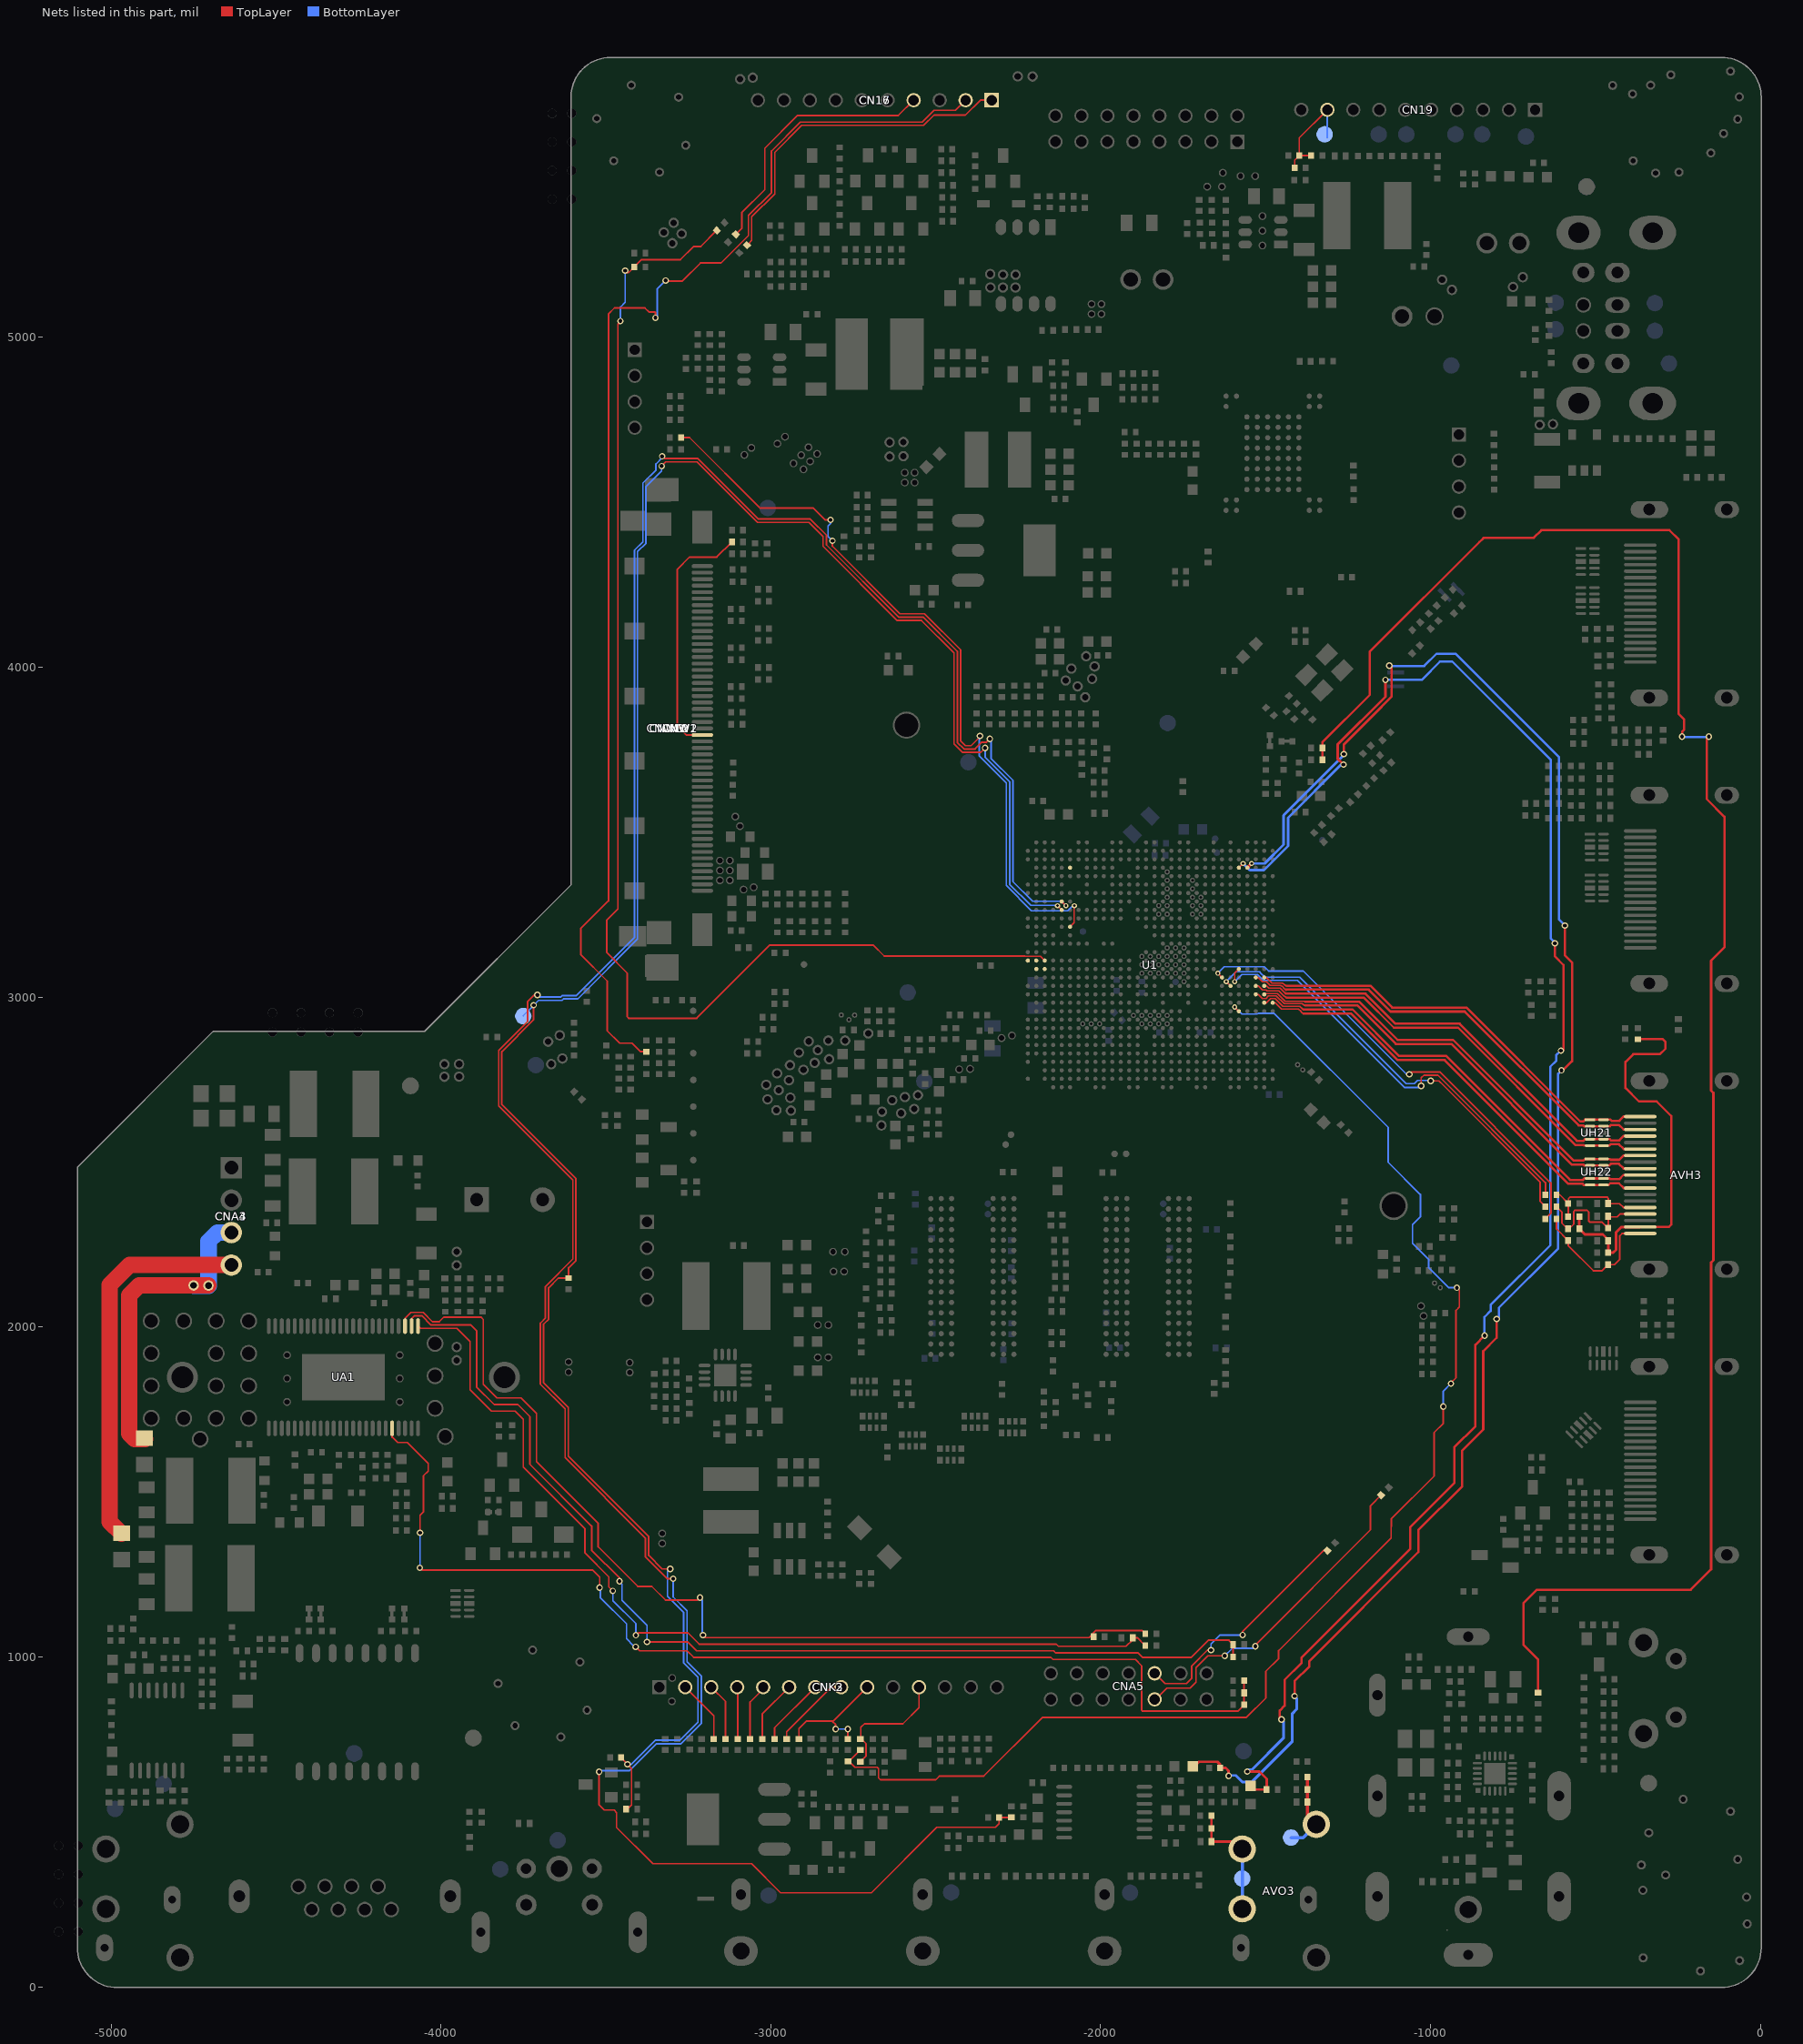
[diagram p0: the nets of this part, all layers, seen from the top]
# Altium PCB MISC86290.PcbDoc (part 23 of 31)
Units mil, origin at the board's own origin, x right, y up, seen from the top; angles counter-clockwise.
Board outline 5104.71 x 5851.49 mil, 2 copper layers (TopLayer, BottomLayer), stack 61.855 mil thick; 1026 components, 667 nets, 4280 pads, 2294 vias.

## Via types
v1: diameter 19.68, hole 11.81, TopLayer to BottomLayer, tented both sides, 1189 vias
v2: diameter 19.68/19.68 (per signal layer), hole 11.81, TopLayer to BottomLayer, tented both sides, 366 vias
v3: diameter 15.75, hole 7.87, TopLayer to BottomLayer, tented both sides, 348 vias
v4: diameter 23.62, hole 15.75, TopLayer to BottomLayer, tented both sides, 309 vias
v5: diameter 15.75/15.75 (per signal layer), hole 7.87, TopLayer to BottomLayer, tented both sides, 59 vias
v6: diameter 24/24 (per signal layer), hole 16, TopLayer to BottomLayer, tented both sides, 23 vias

## Nets (pads, with @x,y where several pads share a name; then routed paths per layer and width w, separated by ;. In a path a pad name is that pad's centre, name@x,y a point inside that pad or via, vN(x,y) a via of type N, cw(c..) or ccw(c..) an arc to the next point about the centre after c; other vN are vias at no path point) (continued)
HDMID-HOTPLUG: RH21.1 U1.P7 | length 1429.1
  TopLayer w3.94: v3(-1645,3072.44) U1.P7@-1632.2,3059.65
  TopLayer w5: v1(-1064.29,2766) -1056.94,2773.35 -972.21,2773.35 -635,2436.15 -635,2344.73 RH21.1@-651.73,2328
  BottomLayer w3.94: v3(-1645,3072.44) -1625.32,3092.13 -1503.82,3092.13 -1501.52,3089.83
  BottomLayer w5: -1501.52,3089.83 -1490.8,3079.11 -1385.61,3079.11 -1072.49,2766 v1(-1064.29,2766)
HDMID-RX0N: AVH3.9 U1.M3 UH22.2 UH22.7 | length 1414.2
  TopLayer w3.94: U1.M3@-1529.84,3008.46 -1522.51,3008.46 -1509.72,2995.67 -1499.19,2995.67 -1491.32,3003.54 -1467.83,3003.54 -1444.21,2979.92 -1391.46,2979.92 cw(c-1391.46,2970.05) -1386.96,2978.84 ; -1384.48,2977.03 ccw(c-1391.46,2970.05) -1385.46,2977.89 ; -1378.29,2975.88 cw(c-1378.29,2989.68) -1385.46,2977.89 ; -1373,2974.58 -1382.71,2974.58 -1386.96,2978.84 ; -1386.96,2978.84 cw(c-1391.46,2970.05) -1386.48,2978.57 ; -1386.48,2978.57 cw(c-1391.46,2970.05) -1385.46,2977.89 ; -1386.48,2978.57 ccw(c-1378.29,2989.68) -1385.46,2977.89
  TopLayer w7: -1380.76,2974.58 -1373,2974.58 -1221.44,2974.58 -1105.21,2858.35 -937,2858.35 -570.89,2492.25 -537,2492.25 -534.44,2489.69 UH22.2@-516.47,2489.69 UH22.7@-475.53,2489.68 -458.13,2489.68 -453,2494.81 -428.92,2494.81 -414.43,2480.32 AVH3.9@-364.47,2480.32
HDMID-RX0P: AVH3.7 U1.M2 UH22.1 UH22.8 | length 1366.6
  TopLayer w3.94: U1.M2@-1504.25,3008.46 -1503.19,3007.4 -1499.17,3011.42 -1463.9,3011.42 -1440.39,2987.91 -1386.58,2987.91 ; -1381.07,2985.63 ccw(c-1386.58,2980.12) -1386.58,2987.91 ; -1379.37,2987.91 -1386.58,2987.91
  TopLayer w7: -1379.9,2986.58 -1216.47,2986.58 -1100.24,2870.35 -932.03,2870.35 -565.92,2504.25 -537,2504.25 -531.87,2509.37 UH22.1@-516.47,2509.37 UH22.8@-475.53,2509.37 -456.56,2509.37 -454,2506.81 -428.08,2506.81 -415.2,2519.69 AVH3.7@-364.47,2519.69
HDMID-RX1N: AVH3.6 U1.N3 UH21.4 UH21.5 | length 1388.1
  TopLayer w3.94: U1.N3@-1529.84,3034.06 -1522.05,3034.06 -1509.64,3021.65 -1498.15,3021.65 -1495.79,3019.29 -1459.96,3019.29 -1443.48,3002.81 ; -1436.82,3000.05 cw(c-1436.82,3009.47) -1443.48,3002.81 ; -1436.25,2999.03 -1439.7,2999.03 ; -1435.7,2997.12 cw(c-1435.7,3002.16) -1439.27,2998.6 -1439.7,2999.03 ; -1443.48,3002.81 -1441.48,3000.81 ; -1441.48,3000.81 -1439.7,2999.03 ; -1441.48,3000.81 -1439.7,2999.03
  TopLayer w7: -1436.25,2998.58 -1202.44,2998.58 -1111.21,2907.35 -916.7,2907.35 -561.54,2552.19 -537,2552.19 -534.44,2549.63 UH21.4@-516.47,2549.63 UH21.5@-475.53,2549.63 -458.24,2549.63 -454,2553.87 -428.92,2553.87 -414.43,2539.37 AVH3.6@-364.47,2539.37
HDMID-RX1P: AVH3.4 U1.N2 UH21.3 UH21.6 | length 1352.1
  TopLayer w3.94: U1.N2@-1504.25,3034.06 -1497.85,3034.06 -1490.96,3027.17 -1456.02,3027.17 -1444.03,3015.17 ; -1436.96,3009.16 cw(c-1436.96,3011.72) -1438.76,3009.9 -1444.02,3015.16 ccw(c-1436.54,3022.66) -1436.54,3012.07
  TopLayer w7: -1437,3010.58 -1197.47,3010.58 -1106.24,2919.35 -911.73,2919.35 -556.57,2564.19 -537,2564.19 -531.87,2569.32 UH21.3@-516.47,2569.32 UH21.6@-475.53,2569.32 -456.45,2569.32 -453,2565.87 -428.08,2565.87 -415.2,2578.74 AVH3.4@-364.47,2578.74
HDMID-RX2N: AVH3.3 U1.P3 UH21.2 UH21.7 | length 1380.6
  TopLayer w3.94: U1.P3@-1529.84,3059.65 -1522.81,3059.65 -1510.01,3046.85 -1497.85,3046.85 -1486.04,3035.04 -1455.54,3035.04 cw(c-1455.54,3026.7) -1449.64,3032.6 -1444.88,3027.84 ; -1436.53,3021.03 -1438.08,3021.03 -1444.88,3027.84 ; -1444.88,3027.84 ccw(c-1435.69,3037.03) -1435.69,3024.03 cw(c-1435.69,3037.03) -1444.88,3027.84
  TopLayer w7: -1436.53,3022.58 -1187.44,3022.58 -1121.21,2956.35 -896.41,2956.35 -551.3,2611.24 -537,2611.24 -534.44,2608.68 UH21.2@-516.47,2608.68 UH21.7@-475.53,2608.68 -456.93,2608.68 -452.69,2612.92 -428.92,2612.92 -414.43,2598.43 AVH3.3@-364.47,2598.43
HDMID-RX2P: AVH3.1 U1.P2 UH21.1 UH21.8 | length 1355.8
  TopLayer w3.94: U1.P2@-1504.25,3059.65 -1497.85,3059.65 -1481.12,3042.91 -1454.24,3042.91 cw(c-1454.24,3028.21) -1443.85,3038.61 ; -1439.98,3034.74 -1443.83,3038.6 ; -1437.69,3036.06 cw(c-1437.69,3044.76) -1443.83,3038.6 ; -1435,3034.58 -1439.81,3034.58 ; -1432.87,3036.02 -1437.6,3036.02 cw(c-1437.6,3044.85) -1443.83,3038.6 ; -1432.11,3033.89 cw(c-1433.73,3035.51) -1433.73,3033.22 -1436.3,3033.22 cw(c-1436.3,3038.43) -1439.81,3034.58 ; -1439.81,3034.58 cw(c-1436.3,3038.43) -1439.97,3034.74 -1439.82,3034.58
  TopLayer w7: -1435,3034.58 -1182.47,3034.58 -1116.24,2968.35 -891.44,2968.35 -546.33,2623.24 -537,2623.24 -531.87,2628.37 UH21.1@-516.47,2628.37 UH21.8@-475.53,2628.37 -454.45,2628.37 -451,2624.92 -428.08,2624.92 -415.2,2637.8 AVH3.1@-364.47,2637.8
HDMID-RXCKN: AVH3.12 U1.L1 UH22.4 UH22.5 | length 1358.7
  TopLayer w3.94: U1.L1@-1478.66,2982.87 -1470.79,2982.87 -1452.09,2964.17 -1400.91,2964.17 -1394.59,2957.86 -1391.54,2954.81 ; -1386.18,2949.44 -1391.53,2954.8 ; -1386.17,2949.44 ccw(c-1385.37,2950.25) -1385.37,2949.11 ; -1384.88,2952.05 cw(c-1384.88,2961.47) -1391.53,2954.8
  TopLayer w7: -1385,2950.58 -1241.11,2950.58 -1099.88,2809.35 -957.29,2809.35 -581.94,2434 -539,2434 -535.63,2430.63 UH22.4@-516.47,2430.63 UH22.5@-475.53,2430.63 -460.13,2430.63 -455,2435.76 -428.92,2435.76 -414.43,2421.26 AVH3.12@-364.47,2421.26
HDMID-RXCKP: AVH3.10 U1.L2 UH22.3 UH22.6 | length 1391.5
  TopLayer w3.94: U1.L2@-1504.25,2982.87 -1503.66,2982.28 -1498.15,2982.28 -1484.76,2995.67 -1471.77,2995.67 -1448.15,2972.05 -1396.55,2972.05 -1391.62,2967.12 ; -1387.08,2962.58 -1387.66,2963.16 ; -1384.18,2964.04 cw(c-1384.18,2974.56) -1391.62,2967.12 ; -1382.47,2961.01 cw(c-1382.47,2968.35) -1387.66,2963.16 ; -1391.62,2967.12 -1387.66,2963.16
  TopLayer w7: -1383.12,2962.58 -1236.14,2962.58 -1094.91,2821.35 -952.32,2821.35 -576.97,2446 -538,2446 -533.69,2450.32 UH22.3@-516.47,2450.32 UH22.6@-475.53,2450.32 -457.56,2450.32 -455,2447.76 -428.08,2447.76 -415.2,2460.63 AVH3.10@-364.47,2460.63
HDMID-SCL_IC: RH25.2 U1.R5 | length 1337.6
  TopLayer w3.94: v3(-1593.82,3046.85) -1593.82,3072.44 U1.R5@-1581.02,3085.24
  TopLayer w5: v1(-1028.5,2731) -1028.5,2755.35 -1020.5,2763.35 -977.38,2763.35 -651.73,2437.7 RH25.2@-651.73,2401
  BottomLayer w3.94: v3(-1593.82,3046.85) -1572.05,3068.61 -1525.31,3068.61 ; -1525.2,3068.5 -1522.25,3065.55
  BottomLayer w5: -1522.25,3065.55 -1507.42,3050.73 -1403.73,3050.73 -1079.3,2726.3 -1033.2,2726.3 v1(-1028.5,2731)
HDMID-SDA_IC: RH26.2 U1.N6 | length 1335
  TopLayer w3.94: v3(-1619.41,3046.85) U1.N6@-1606.61,3034.06
  TopLayer w5: v1(-999.5,2746) -974.17,2746 -961.17,2733 -668.09,2439.92 -668.09,2380.75 ; -667.73,2381 RH26.2@-651.73,2365
  BottomLayer w3.94: v3(-1619.41,3046.85) -1589.81,3076.45 -1518.14,3076.45 -1514.72,3073.03
  BottomLayer w5: -1514.72,3073.03 -1501.88,3060.19 -1396.19,3060.19 -1073.7,2737.7 -1049.07,2737.7 -1039.53,2747.24 -1000.74,2747.24 v1(-999.5,2746)
HDMID_5V: AVH3.18 CH22.1 DH22.K RH22.2 RH23.2 RH24.2 | length 1259.9
  TopLayer w7: RH22.2@-372,2872.27 -296.27,2872.27 -288,2864 -288,2844 -305,2827 -385.44,2827 -409,2803.44 -409,2724.56 -368.44,2684 -314.79,2684 -270.66,2639.86 -270.66,2310.34 -277.85,2303.15 AVH3.18@-364.47,2303.15
  TopLayer w8: RH24.2@-549.27,2334 RH23.2@-549.27,2298 -532.27,2281 -478,2281 -461.27,2264.27 DH22.K@-461.27,2261 CH22.1@-461.27,2226 -446,2226 -438,2234 -438,2287 -421.85,2303.15 AVH3.18@-364.47,2303.15
HDMID_HPD: AVH3.19 CH21.1 DH21.K RH21.2 | length 434.3
  TopLayer w5: RH21.2@-618.27,2328 -618.27,2297.54 CH21.1@-582.73,2262 -582.73,2246.71 -506.7,2170.67 -479.59,2170.67 DH21.K@-461.27,2189 -442.57,2189 -426.5,2205.07 -426.5,2276.5 -419.53,2283.47 AVH3.19@-364.47,2283.47
HDMID_SCL: AVH3.15 CH24.1 DH24.K RH24.1 RH25.1 | length 343.5
  TopLayer w5: RH25.1@-618.27,2401 -608.63,2401 -582.73,2375.1 CH24.1@-582.73,2374 ; RH24.1@-582.73,2334 CH24.1@-582.73,2373 ; CH24.1@-581.73,2374 -581.73,2389.27 -577,2394 -465,2394 -461.27,2390.27 DH24.K@-461.27,2374 -427,2374 -415.21,2362.21 AVH3.15@-364.47,2362.21
HDMID_SDA: AVH3.16 CH23.1 DH23.K RH23.1 RH26.1 | length 426.3
  TopLayer w5: RH26.1@-618.27,2365 -601.91,2348.64 -601.91,2315.18 -583.73,2297 RH23.1@-582.73,2296 ; RH23.1@-579,2296 -579,2298 -579,2299 -566,2312 -566,2350 -562,2354 -526,2354 -520,2348 -520,2321 -516.67,2317.67 -479.67,2317.67 -461.63,2299.63 CH23.1@-461.27,2299.27 ; CH23.1@-461.27,2296 CH23.1@-461.27,2299.27 ; AVH3.16@-364.47,2342.52 -426,2342.52 -434.52,2334 -461.27,2334 CH23.1@-461.27,2300 CH23.1@-461.27,2299.27
HOST_WAKE_WL: CN19.9 CU11.1 HOST_WAKE_WL.1 RU11.1 RU17.1 | length 338.8
  TopLayer w5: RU17.1@-1411.73,5514 -1411.73,5537.54 CU11.1@-1398.27,5551 ; RU11.1@-1361.73,5551 CU11.1@-1398.27,5551 ; CN19.9@-1313.15,5690.24 -1398.27,5605.12 CU11.1@-1398.27,5551
  BottomLayer w5: HOST_WAKE_WL.1@-1313.15,5605 CN19.9@-1313.15,5690.24
HP_AU_LOUT: CO12.2 CO14.2 U1.AG5 | length 5099.2
  TopLayer w4.92: U1.AG5@-1581.02,3392.32 v3(-1568.23,3405.12)
  TopLayer w7: v1@-1457,815 -1457,837.32 -1442.5,851.82 -1442.5,930.14 -1391.66,980.98 -1391.66,996.97 -1061.09,1327.54 -1061.09,1393.85 -928.28,1526.65 -928.28,1635.34 -864.34,1699.27 -864.34,1945.66 v1(-836,1974) ; v1(-623,3163) -623,3123.24 -597,3097.24 v1@-597,2841
  TopLayer w8: v1@-1555.57,652.43 v1(-1555.57,652.16) -1555.41,652 -1519.05,652 -1497,629.95 CO12.2@-1497,597.85 -1534.54,597.85 CO14.2@-1545.5,608.81 ; v1(-1264,3705) -1282,3723 -1282,3765.52 -1137,3910.52 v1(-1137,3962)
  BottomLayer w7: v1(-1137,3962) -1026.91,3962 -971.57,4017.34 -934.37,4017.34 -635.34,3718.31 -635.34,3177.34 v1@-623,3165 ; v1@-836.34,1974.34 -836.34,2030.39 -817.94,2048.79 -817.94,2067.06 -637,2248 -637,2788.97 -619.34,2806.63 -619.34,2823.66 v1(-605,2838)
  BottomLayer w8: v3(-1568.23,3405.12) -1548.22,3385.11 -1504.89,3385.11 -1432,3458 -1432,3544.12 v1@-1271.12,3705 ; v1@-1555.57,658 -1541.46,658 -1446.16,753.3 v1@-1446.16,804.16
  other v1: -1452,810
HP_AU_ROUT: CO11.2 CO13.2 U1.AG4 | length 5262.1
  TopLayer w7: v1(-1412.16,881.2) -1412.16,926.54 -1367.49,971.21 -1367.49,987.2 -1037.09,1317.6 -1037.09,1383.91 -904.28,1516.71 -904.28,1625.39 -840.34,1689.33 -840.34,1926.6 -799.62,1967.32 v1(-799.62,2024.2) ; -1148.07,3881.07 -1118.34,3910.79 -1118.34,3998.34 v1(-1125,4005) ; v1(-603,2778) -599,2778 -571,2806 -571,3105.18 -592.34,3126.52 -592.34,3216.34 v1(-593,3217)
  TopLayer w8: CO13.2@-1720.88,668.5 -1715.5,668.5 -1702.16,681.84 -1646.02,681.84 ; -1658.89,681.82 -1646,681.82 -1638.04,673.85 CO11.2@-1638.04,663.01 -1621,663 -1612,654 v1(-1612,639) ; v1@-1415.36,878 v1(-1412.16,881.2) ; v1(-1263,3737) -1263,3766.13 -1148.07,3881.07
  TopLayer w10: U1.AG4@-1555.43,3392.32 v3(-1542.64,3405.12)
  BottomLayer w7: v1(-1125,4005) -1124,4004 -1019,4004 -981.66,4041.34 -924.43,4041.34 -611.34,3728.25 -611.34,3236.34 -593,3218 v1(-593,3217) ; v1@-796.41,2021 v1(-799.62,2024.2) -793,2030.82 -793,2058.06 -613,2238.06 -613,2768 v1(-603,2778)
  BottomLayer w8: v1(-1612,639) -1610.5,640.5 -1590.38,640.5 -1569.88,620 -1542.69,620 -1419,743.69 -1419,828 -1405.32,841.68 -1405.32,874.36 v1(-1412.16,881.2) ; v3(-1542.64,3405.12) -1502.88,3405.12 -1446,3462 -1446,3551.11 -1263,3734.11 v1(-1263,3737)
HP_DET: CO24.2 HP_DET.1 RO22.2 RO28.2 U1.AB26 | length 7101.6
  TopLayer w3.94: v3(-2131.22,3277.17) U1.AB26@-2118.43,3264.37
  TopLayer w5: v1(-3719,2975.5) -3719,2931.66 -3815.8,2834.86 -3815.8,2674.19 -3591.05,2449.44 -3591.05,2201.59 -3613,2179.64 CO24.2@-3613,2148.23 -3644.41,2148.23 -3673.68,2118.96 -3673.68,2024.09 -3688.8,2008.96 -3688.8,1830.53 -3613.8,1755.53 -3613.8,1608.1 -3370.34,1364.64 -3370.34,1307.34 -3329.5,1266.5 v1(-3305,1266.5) ; RO22.2@-3453.54,695 -3453.54,694.18 -3434.5,675.14 v1(-3434.5,674) -3422,661.5 -3422,550.99 -3434.46,538.53 RO28.2@-3438.52,538.53 ; v1(-3331,4610) -3318.34,4622.66 -3224.14,4622.66 -3040.83,4439.34 -2884.87,4439.34 -2841.5,4395.97 -2841.5,4366.97 -2616.53,4142 -2543.14,4142 -2444.5,4043.36 -2444.5,3767.95 -2418.66,3742.11 -2363.95,3742.11 v1(-2350.61,3755.45)
  BottomLayer w5: HP_DET.1@-3750.5,2942.5 -3750.5,2944 v1(-3719,2975.5) -3704.16,2990.34 -3632.87,2990.34 -3628.2,2995.01 -3585.03,2995.01 -3404.11,3175.94 -3404.11,4350.52 -3378.5,4376.13 -3378.5,4548 -3331,4595.5 v1(-3331,4610) ; v1@-3434.5,673.74 -3423.26,673.74 -3350,747 -3276,747 -3220.73,802.27 -3220.73,938.09 -3264.25,981.61 -3264.25,1134.25 -3313.43,1183.43 -3313.43,1258.07 v1(-3305,1266.5) ; v1(-2350.61,3755.45) -2350.61,3727.72 -2276,3653.11 -2276,3342.11 -2211.92,3278.03 v3@-2132.09,3278.03
HP_MUTEN: RO29.1 RO30.2 U1.AC26 | length 8640.8
  TopLayer w3.94: U1.AC26@-2118.43,3289.96 v3(-2105.63,3277.17)
  TopLayer w5: v1(-3707.54,3006.58) -3716.92,3006.58 -3737.5,2986 -3737.5,2925.75 -3824.7,2838.55 -3824.7,2670.5 -3599.95,2445.75 -3599.95,2206.13 -3683.18,2122.9 -3683.18,2027.18 -3698.8,2011.55 -3698.8,1826.39 -3623.8,1751.39 -3623.8,1603.96 -3380.34,1360.5 -3380.34,1303.2 -3313.76,1236.62 v1(-3296.09,1236.62) ; v1(-3520.5,651.43) -3520.5,551 -3505,535.5 -3475.07,535.5 -3467.57,528 -3467.57,482.57 -3358,373 -3058.73,373 -2970.73,285 -2695,285 -2496.66,483.34 -2319.66,483.34 -2308.27,494.73 RO30.2@-2308.27,513 RO29.1@-2271.27,513 ; v1@-3322.66,4632.66 -3221.41,4632.66 -3038.1,4449.34 -2880.73,4449.34 -2831.5,4400.11 -2831.5,4371.11 -2612.39,4152 -2538.14,4152 -2434.5,4048.36 -2434.5,3772.09 -2414.52,3752.11 -2380.89,3752.11 -2360.2,3772.8 -2346.32,3772.8 v1(-2336,3783.11)
  BottomLayer w3.94: -2141.81,3290.94 -2119.41,3290.94 v3(-2105.63,3277.17)
  BottomLayer w5: v1(-3707.54,3006.58) -3701.3,3000.34 -3637.01,3000.34 -3632.34,3005.01 -3589.18,3005.01 -3413.61,3180.58 -3413.61,4354.45 -3388,4380.07 -3388,4558.5 -3348.34,4598.16 -3348.34,4616.48 v1@-3329.5,4635.32 ; v1(-3520.5,651.43) -3517.18,654.75 -3429.25,654.75 -3348,736 -3272.86,736 -3210.73,798.13 -3210.73,942.23 -3254.25,985.75 -3254.25,1139.89 -3296.09,1181.74 v1(-3296.09,1236.62) ; v1@-2332.68,3779.8 -2332.68,3723.94 -2266,3657.25 -2266,3350.37 -2206.57,3290.94 -2141.81,3290.94
  other v1: -3329.5,4639.5
HP_OUT_L: AVO3.4 AVO3.5 DO12.K HP_OUT_L.1 RO16.2 RO25.2 | length 387.6
  TopLayer w8: RO16.2@-1664.27,518 DO12.K@-1664.27,440 -1593.55,440 AVO3.5@-1570.87,417.32 AVO3.5@-1596.59,417.32
  BottomLayer w10: AVO3.4@-1570.87,236.22 HP_OUT_L.1@-1570.87,328 AVO3.5@-1570.87,417.32
HP_OUT_R: AVO3.3 DO11.K HP_OUT_R.1 RO15.2 RO24.2 | length 274.1
  TopLayer w10: -1373.67,543.47 RO24.2@-1373.67,597.86 RO15.2@-1373.67,635.36 ; DO11.K@-1373.27,559.5 -1373.27,500.89 -1364.5,492.13 AVO3.3@-1346.46,492.13
  BottomLayer w10: HP_OUT_R.1@-1423,452 -1386.59,452 AVO3.3@-1346.46,492.13
HTPDN_TX: CNW1.27 CNW2.27 CNW3.27 CNW12.27 RW11.1 | length 766.6
  TopLayer w5: CNW3.27@-3207.67,3794.84 -3256.23,3794.84 -3283.5,3822.11 -3283.5,4296.89 -3246.4,4334 -3164.01,4334 -3118,4380 RW11.1@-3117.71,4380 RW11.1@-3117.71,4375.53
I2S_BCK_A: DA2.K RA3.2 UA1.26 | length 3298.5
  TopLayer w5: UA1.26@-4089.06,2002.77 -4089.06,2024.94 -4080,2034 -4058,2034 -4030,2006 -3909,2006 -3892,1989 -3892,1818.57 -3838.43,1765 -3767.14,1765 -3730.5,1728.36 -3730.5,1583.93 -3543.25,1396.68 -3543.25,1322.96 -3458.68,1238.4 v1(-3458.68,1229.21) ; v1(-3375.5,1045.5) -3252.7,1045.5 -3225.52,1018.31 -2142.74,1018.31 -2136.43,1012 -1886.18,1012 -1872.18,998 -1726.71,998 -1674.1,1050.61 -1612.34,1050.61 ; -1611.34,1050.61 DA2.K@-1598.23,1037.5 ; RA3.2@-1598.73,1000 DA2.K@-1598.73,1037
  BottomLayer w5: v1@-3458.68,1226.68 -3451.34,1219.34 -3451.34,1170.99 -3375.5,1095.15 v1(-3375.5,1045.5)
I2S_IN_BCK: U1.R29
I2S_IN_D0: U1.T30
I2S_IN_D1: U1.T29
I2S_IN_WCK: U1.R28
I2S_LRCLK_A: DA5.K RA2.2 UA1.25 | length 2895.4
  TopLayer w5: UA1.25@-4069.37,2002.77 -4062.61,1996 -3952,1996 -3912,1956 -3912,1810.29 -3846.71,1745 -3775.43,1745 -3750.5,1720.07 -3750.5,1575.64 -3563.25,1388.39 -3563.25,1314.68 -3491,1242.43 -3491,1212 v1(-3479,1200) ; -3401.5,1073 -3251.92,1073 -3217.23,1038.31 -2134.46,1038.31 -2128.14,1032 -1923.17,1032 -1903.27,1051.91 DA5.K@-1903.27,1058 -1888.73,1058 RA2.2@-1864.73,1034
  BottomLayer w5: v1(-3479,1200) -3479,1170.37 -3409,1100.37 v1(-3409,1065.5)
I2S_MCK_A: CA29.2 DA1.K RA4.2 UA1.20 | length 3382.2
  TopLayer w5: -4148.11,1666.54 -4131.58,1650 -4102.11,1650 -4038.66,1586.54 -4038.66,1563.32 -4053.5,1548.47 -4053.5,1439.36 -4063.5,1429.36 v1(-4063.5,1376) ; v1(-4064,1270) -4056.66,1262.66 -3539.52,1262.66 -3519,1242.14 v1(-3519,1210) ; v1(-3410,1030.5) -3397.66,1018.16 -3253.64,1018.16 -3233.8,998.31 -2151.02,998.31 -2144.71,992 -1895,992 -1875.85,972.85 -1875.85,837.99 -1873.36,835.5 -1584.77,835.5 CA29.2@-1565.27,855 ; CA29.2@-1565.27,855.73 DA1.K@-1565.27,891 RA4.2@-1565.27,928
  TopLayer w6: -4148.11,1666.54 UA1.20@-4148.11,1688.79
  BottomLayer w5: v1(-4064,1270) -4063.5,1270.5 v1(-4063.5,1376) ; v1@-3517,1209 -3517,1180.08 -3437.28,1100.36 -3437.28,1055.11 v1@-3416.17,1034
I2S_OUT_SD1: CNA5.5 R135.2 | length 752.4
  TopLayer w5: CNA5.5@-1836.26,950 -1805.26,919 -1740,919 -1724,935 -1724,972.43 -1676.13,1020.3 v1(-1665.74,1020.3) ; CNA5.5@-1836.26,962 CNA5.5@-1826,962 ; v1(-1570.04,1066.29) -1570.04,1076.68 -1324.54,1322.17 R135.2@-1312.83,1322.17
  BottomLayer w5: v1(-1665.74,1020.3) -1665.74,1038.87 -1638.32,1066.29 v1(-1570.04,1066.29)
I2S_OUT_SD2: CNA5.6 R136.2 | length 1016.6
  TopLayer w4.92: CNA5.6@-1836.26,875.26 -1830,875.26 -1799.76,905.5 -1728.5,905.5 -1711,923 -1711,967 -1675,1003 v1(-1624,1003) ; v1(-1531,1032) -1531,1036.77 -1182.05,1385.72 -1182.05,1457.95 R136.2@-1146.6,1493.4
  BottomLayer w4.92: v1(-1624,1003) -1601,1026 -1537,1026 v1(-1531,1032)
I2S_SD_A: DA6.K RA1.2 UA1.27 | length 3015
  TopLayer w5: UA1.27@-4108.74,2002.77 -4108.74,2026.26 -4091,2044 -4053.86,2044 -4025.86,2016 -4005,2016 -3991.09,2029.91 -3879,2029.91 -3872,2022.91 -3872,1826.86 -3830.14,1785 -3757.14,1785 -3710.5,1738.36 -3710.5,1592.21 -3523.25,1404.96 -3523.25,1333.48 -3403.28,1213.5 -3360.93,1213.5 -3319.43,1172 -3222,1172 v1(-3214.5,1179.5) ; v1(-3205.91,1065.66) -3198.56,1058.31 -2035.69,1058.31 -2014,1080 -1874.73,1080 RA1.2@-1864.73,1070
  BottomLayer w5: v1(-3214.5,1179.5) -3208,1173 v1@-3208,1067.75
IF_AGC/: CT13.2 RT1.1 RT9.2 | length 5660.5
  TopLayer w7: RT1.1@-1328.27,3719.5 CT13.2@-1328.27,3755.5 -1328.27,3772.28 -1183.77,3916.78 -1183.77,4047.89 ; -1167.36,4064.3 -1183.77,4047.89 ; RT9.2@-674,891.23 -674,991.5 -718.84,1036.34 -718.84,1162.41 -678.01,1203.25 -211.59,1203.25 -149.5,1265.34 -149.5,2195.56 -142.66,2202.4 -142.66,2709.6 -149.5,2716.44 -149.5,3110.32 -109,3150.82 -109,3547 -163,3601 v1@-163,3783.34 ; v1(-237.5,3790) -237.5,3804.5 -231,3811 -231,3841.94 -247.5,3858.44 -247.5,4387.5 -275.7,4415.7 -663.98,4415.7 -687.18,4392.5 -839.16,4392.5 -840.85,4390.82 -851.59,4380.07 -1183.77,4047.89
  BottomLayer w7: v1@-235.5,3788 v1@-158.34,3788
  other v1: -156.66,3789.68
IR_IN: CNK2.11 CNK3.11 RK1.1 RK2.1 | length 382.9
  TopLayer w5: RK1.1@-2728.5,682.73 -2711.16,700.07 -2711.16,736.34 -2725.55,750.73 RK2.1@-2727.25,750.73 ; RK2.1@-2728.5,750.73 RK2.1@-2727.25,750.73 ; CNK2.11@-2550.72,908 -2550.72,846.06 -2599.78,797 -2716.5,797 -2727.25,786.25 RK2.1@-2727.25,750.73
IR_IN_IC: CK1.2 RK2.2 U1.K5 | length 4197.3
  TopLayer w3.94: v3(-1593.82,2970.08) U1.K5@-1581.02,2957.28
  TopLayer w5: CK1.2@-2766,682.73 CK1.2@-2763.04,682.73 ; RK2.2@-2728.5,717.27 CK1.2@-2763.04,682.73 ; -1119.59,1404 -1119.59,1359.85 -1460.5,1018.94 -1460.5,994.87 -1499.5,955.87 -1499.5,875.43 -1558.93,816 -2177,816 -2354.5,638.5 -2489.16,638.5 -2500.32,627.34 -2667.84,627.34 -2673.5,633 -2673.5,661 -2677.98,665.48 -2745.78,665.48 CK1.2@-2763.04,682.73 ; -1119.09,1395 -1119.09,1417.87 -989.3,1547.66 -989.3,1679.74 -961.32,1707.73 v1(-961.32,1758.59) ; v1@-938.5,1830.5 -923,1846 -923,2050 -912.5,2060.5 -912.5,2111.5 v1(-920,2119)
  BottomLayer w3.94: v3(-1593.82,2970.08) -1572.17,2948.43 -1526.83,2948.43 -1524.72,2950.53 -1522.22,2950.53
  BottomLayer w5: -1522.22,2950.53 -1474.03,2950.53 -1128.51,2605.01 -1128.51,2499.17 -1031,2401.66 -1031,2334.14 -1054.99,2310.15 -1054.99,2253.51 -1005.66,2204.18 -1005.66,2179.76 -944.9,2119 v1(-920,2119) ; v1(-961.32,1758.59) -961.32,1805.68 v1(-938.5,1828.5)
K0/AD: CNK2.9 CNK3.9 RK35.2 RK41.2 | length 385.5
  TopLayer w5: RK35.2@-2914.88,751 -2914.88,783.12 -2893,805 -2813.73,805 ; v1(-2803.5,781.02) -2803.5,794.77 -2813.73,805 ; RK41.2@-2766.5,751.23 v1(-2766.5,781.02) ; CNK2.9@-2708.2,908 -2811.2,805 -2813.73,805
  BottomLayer w5: v1(-2803.5,781.02) v1(-2766.5,781.02)
K1: CNK2.8 CNK3.8 RK27.2 | length 243
  TopLayer w5: RK27.2@-2951.94,751 -2951.94,773.06 -2817,908 CNK2.8@-2786.94,908
K2: CNK2.7 CNK3.7 RK28.2 | length 208.1
  TopLayer w5: RK28.2@-2989,751 -2989,784.68 CNK2.7@-2865.68,908
K3: CNK2.6 CNK3.6 RK29.2 | length 190.8
  TopLayer w5: RK29.2@-3026.07,751 -3026.07,826.36 CNK2.6@-2944.42,908
K4: CNK2.5 CNK3.5 RK30.1 | length 173.6
  TopLayer w5: RK30.1@-3063.13,751 -3063.13,862.87 -3023.16,902.84 CNK2.5@-3023.16,908
K5: CNK2.4 CNK3.4 RK31.2 | length 157
  TopLayer w5: CNK2.4@-3101.9,906.29 CNK2.4@-3101.9,908 ; RK31.2@-3100.19,751 CNK2.4@-3100.19,906.29
K6/AD: CNK2.3 CNK3.3 RK36.2 | length 175
  TopLayer w5: CNK2.3@-3180.64,908 -3137.25,864.61 RK36.2@-3137.25,751
K7: CNK2.2 CNK3.2 RK32.2 | length 190.4
  TopLayer w5: CNK2.2@-3257.63,906.25 -3172.88,821.49 RK32.2@-3172.88,751
L_OUT+: CNA3.4 CNA4.4 RA30.2 | length 1161.7
  TopLayer w50: RA30.2@-4969,1374.09 -5004.17,1409.27 -5004.17,2127.77 -4944.13,2187.81 CNA4.4@-4635.54,2187.81
L_OUT-: CNA3.3 CNA4.3 pad.VIA5@-4704.69,2125.6 pad.VIA5@-4750,2126 RA31.2 | length 984.5
  TopLayer w50: RA31.2@-4897.01,1660.09 -4899.01,1660.09 -4928.09,1660.09 -4945,1677 -4945,2095.73 -4914.73,2126 pad.VIA5@-4750,2126 pad.VIA5@-4705.73,2126
  BottomLayer w50: pad.VIA5@-4749.6,2125.6 pad.VIA5@-4704.69,2125.6 -4704.69,2259.31 -4677.77,2286.23 CNA4.3@-4635.54,2286.23
LCD_EN: CN16.1 CN17.1 RG42.1 | length 1033.3
  TopLayer w5: RG42.1@-3068,5283.73 -3058.09,5293.64 -3058.09,5365.34 -2988,5435.43 -2988,5560.93 -2906.09,5642.85 -2536.48,5642.85 -2505.32,5674 -2410,5674 -2364.54,5719.46 CN16.1@-2330.67,5719.46
LD_EN-SET_MOD: U1.AG25
LD_GPIO: RG44.2 U1.Y25 | length 2322.9
  TopLayer w3.9: U1.Y25@-2092.83,3213.19 -2080.04,3225.98 v3(-2080.04,3277.17)
  TopLayer w3.94: U1.Y25@-2092.83,3213.19 U1.Y25@-2090.08,3213.19
  TopLayer w5: RG44.2@-3272.54,4696.5 -3246.44,4696.5 -3032.94,4483 -2871.96,4483 -2835.96,4447 v1(-2819.25,4447) ; v1(-2813.18,4383.31) -2813.18,4366.94 -2608.25,4162 -2534,4162 -2424.5,4052.5 -2424.5,3776.24 -2410.37,3762.11 -2393,3762.11 -2366,3789.11 v1(-2366,3792.11)
  BottomLayer w3.94: -2286,3359.11 -2286,3338.72 -2209.6,3262.32 -2099.48,3262.32 -2084.64,3277.17 v3(-2080.04,3277.17)
  BottomLayer w5: v1(-2819.25,4447) -2819.25,4435.34 -2826.59,4428 -2826.59,4396.72 v1(-2813.18,4383.31) ; v1(-2366,3792.11) -2367.95,3790.16 -2367.95,3730.92 -2286,3648.97 -2286,3359.11
LD_HSYNC: R130.1 RG41.2 U1.T28 | length 4029.3
  TopLayer w3.94: -2182.4,3123.62 U1.T28@-2169.61,3110.83
  TopLayer w5: -3463.61,5041.94 -3463.61,3267.53 -3497.13,3234.01 -3497.13,3134.71 -3435.34,3072.92 -3435.34,2940.34 -3431,2936 -3224.51,2936 -3002.51,3158 -2689.71,3158 -2656.21,3124.5 -2229.48,3124.5 -2228.6,3123.62 -2182.4,3123.62 ; -3463.11,5038.93 -3455.77,5046.27 v1(-3455.77,5049.78) ; v1(-3441.5,5202.5) -3441.5,5196.5 -3431.23,5196.5 R130.1@-3413.73,5214 R130.1@-3409.5,5218.23 ; R130.1@-3409.63,5218.37 -3392.16,5235.84 -3274,5235.84 -3233.85,5276 -3212,5276 RG41.2@-3163.83,5324.17
  BottomLayer w5: v1(-3455.77,5049.78) -3455.77,5092.23 -3441.66,5106.34 -3441.66,5202.34 v1(-3441.5,5202.5)
LD_SPI_CLK: CN16.4 CN17.4 R129.2 | length 809.2
  TopLayer w5: R129.2@-3106.17,5312.33 -3088.09,5330.41 -3088.09,5377.76 -3018,5447.85 -3018,5573.36 -2918.51,5672.85 -2613.5,5672.85 CN16.4@-2566.89,5719.46
LD_SPI_CSZ: CN16.2 CN17.2 R127.2 | length 3939.5
  TopLayer w5: R127.2@-3377,2834.77 -3394.77,2834.77 -3420.5,2860.5 -3458.5,2860.5 -3496,2898 -3496,3048.65 -3576.16,3128.81 -3576.16,3207.69 -3492.11,3291.75 -3492.11,5071.28 -3473.89,5089.5 -3382,5089.5 -3369.91,5077.41 -3352.41,5077.41 -3349.71,5074.71 v1(-3349.71,5059.44) ; v1(-3319,5172.5) v1@-3312,5172.5 ; v1@-3317.5,5171 -3268.14,5171 -3213.14,5226 -3150.86,5226 -3068.09,5308.77 -3068.09,5369.48 -2998,5439.57 -2998,5565.07 -2910.23,5652.85 -2540.62,5652.85 -2504.96,5688.5 -2440.37,5688.5 CN16.2@-2409.41,5719.46
  BottomLayer w5: v1(-3349.71,5059.44) -3344,5065.15 -3344,5147.5 v1(-3319,5172.5) v1@-3319,5168